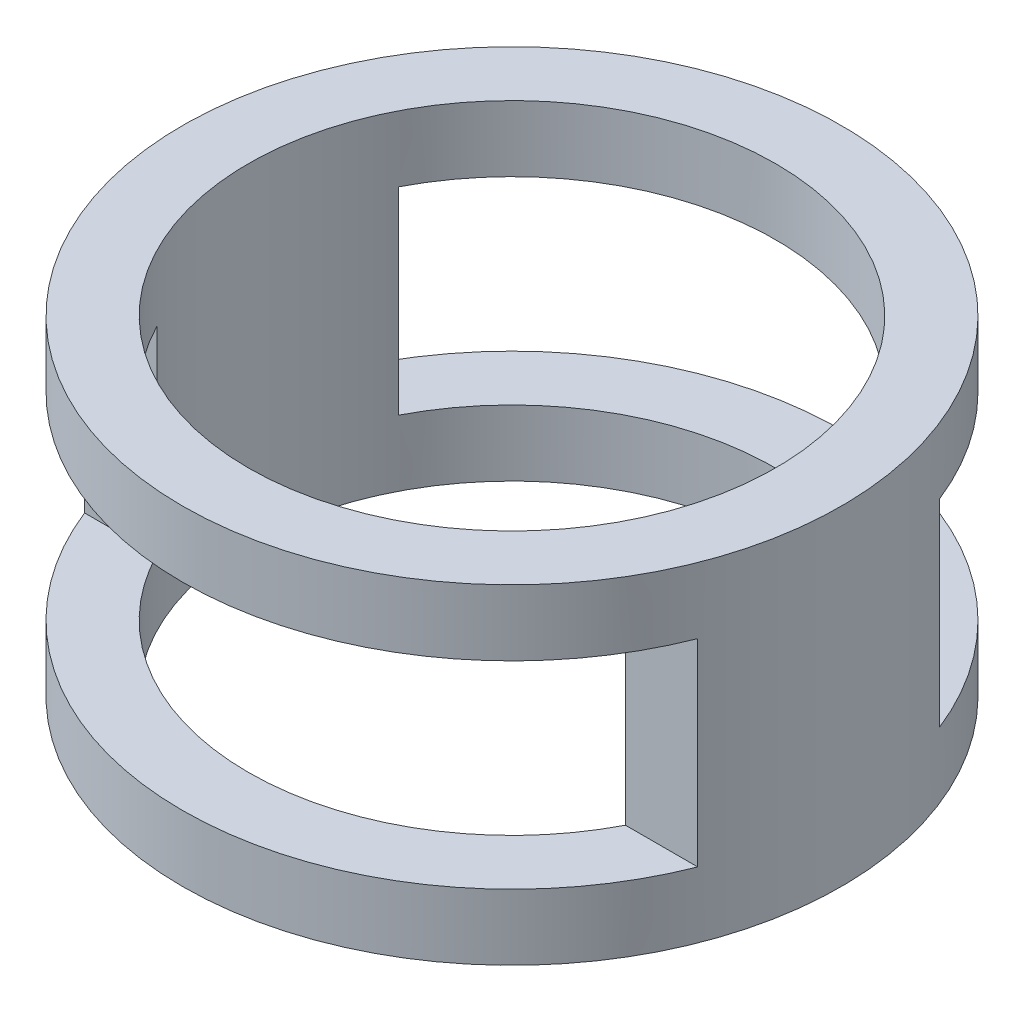
from build123d import *

# Parameters (mm, degrees)
SKETCH1_R               = 30
SKETCH1_R_2             = 24
BOSS_EXTRUDE1_DEPTH     = 30
CUT_EXTRUDE1_DEPTH      = 52.961524227
CUT_EXTRUDE1_DEPTH_BACK = 52.961524227
SKETCH2_W               = 38
SKETCH2_H               = 18


with BuildPart() as part:
    # Sketch1 → Boss-Extrude1 (new body)
    with BuildSketch(Plane(origin=(0, 0, 0), x_dir=(1, 0, 0), z_dir=(0, 1, 0))):
        with Locations(Location((0, 0, 0), (0, 0, 270))):
            Circle(SKETCH1_R)
        with Locations(Location((0, 0, 0), (0, 0, 270))):
            Circle(SKETCH1_R_2, mode=Mode.SUBTRACT)
    extrude(amount=BOSS_EXTRUDE1_DEPTH)

    # Sketch2 → Cut-Extrude1 (cut, two sides: drawn at the far end of the back side and taken through both)
    with BuildSketch(Plane(origin=(0, 0, 0), x_dir=(0, 0, -1), z_dir=(1, 0, 0)).offset(-CUT_EXTRUDE1_DEPTH_BACK)):
        with Locations((-30, 15)):
            Rectangle(SKETCH2_W, SKETCH2_H)
        with Locations((30, 15)):
            Rectangle(SKETCH2_W, SKETCH2_H)
    extrude(amount=CUT_EXTRUDE1_DEPTH + CUT_EXTRUDE1_DEPTH_BACK, mode=Mode.SUBTRACT)


solid = part.part
